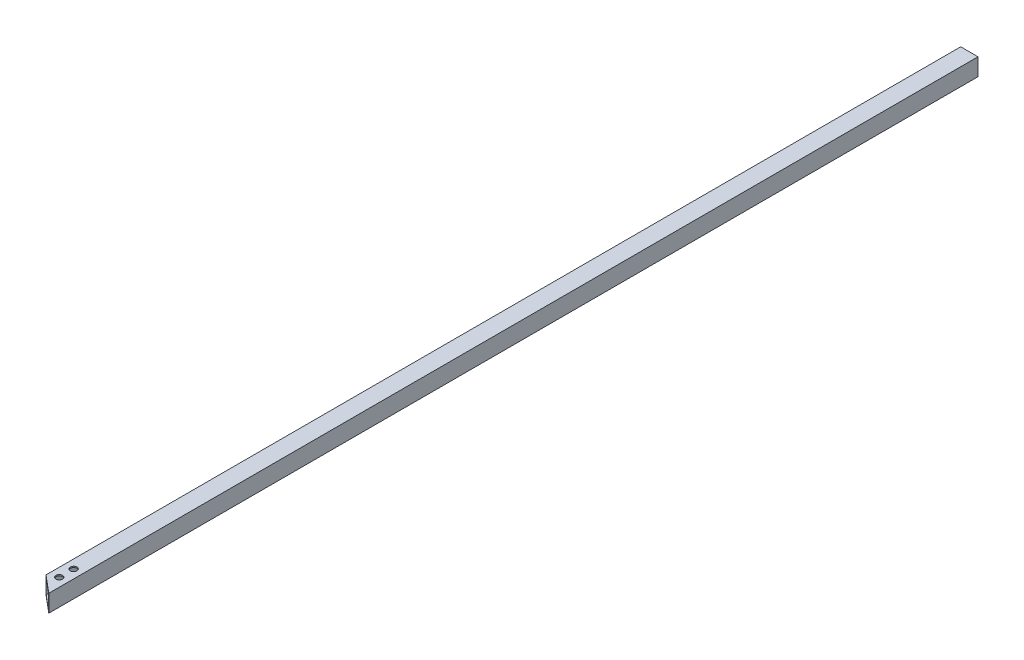
from build123d import *

# Parameters (mm, degrees)
SKETCH_1_W          = 30
SKETCH_1_H          = 30
SKETCH_1_W_2        = 26
SKETCH_1_H_2        = 26
EXTRUDE_1_DEPTH     = 833.5
CUT_EXTRUDE_1_DEPTH = 35
SKETCH_4_R          = 5.75
CUT_EXTRUDE_2_DEPTH = 163


with BuildPart() as part:
    # 草图1 → 凸台-拉伸1 (new, symmetric)
    with BuildSketch(Plane.XY):
        Rectangle(SKETCH_1_W, SKETCH_1_H)
        Rectangle(SKETCH_1_W_2, SKETCH_1_H_2, mode=Mode.SUBTRACT)
    extrude(amount=EXTRUDE_1_DEPTH, both=True)

    # 草图3 → 切除-拉伸1 (cut, symmetric)
    with BuildSketch(Plane(origin=(0, 15, 0), x_dir=(1, 0, 0), z_dir=(0, 1, 0))):
        Polygon((15, -833.5), (15, -778.5), (-15, -753.327011065), (-15, -833.5), align=None)
    extrude(amount=CUT_EXTRUDE_1_DEPTH, both=True, mode=Mode.SUBTRACT)

    # 草图4 → 切除-拉伸2 (cut)
    with BuildSketch(Plane.XZ.offset(15)):
        with Locations((0, 745.413505532)):
            Circle(SKETCH_4_R)
        with Locations((0, 720.413505532)):
            Circle(SKETCH_4_R)
    extrude(amount=-CUT_EXTRUDE_2_DEPTH, mode=Mode.SUBTRACT)


solid = part.part
